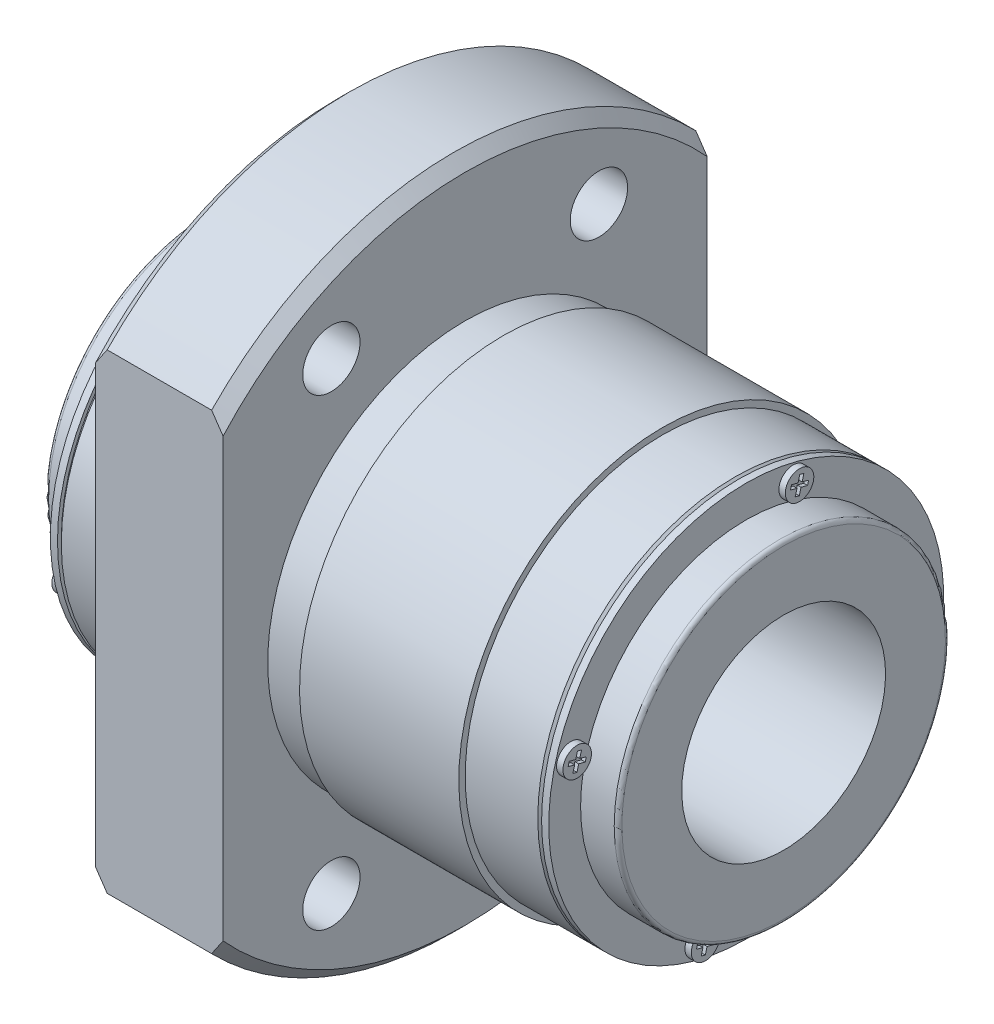
from build123d import *

# Parameters (mm, degrees)
SKETCH2_OUTSIDE_W          = 72.484
SKETCH2_OUTSIDE_H          = 72.484
SKETCH2_OUTSIDE_W_2        = 38
SKETCH2_OUTSIDE_H_2        = 53
CUT_EXTRUDE1_DEPTH         = 52.278650528
F_4_5_4_5_DIAMETER_HOLE1_D = 4.5
SKETCH6_R                  = 1.12
BOSS_EXTRUDE1_DEPTH        = 0.5
CUT_EXTRUDE2_DEPTH         = 0.3
CIRPATTERN1_COUNT          = 4
SKETCH8_R                  = 1.12
BOSS_EXTRUDE2_DEPTH        = 0.5
CUT_EXTRUDE3_DEPTH         = 0.3
CIRPATTERN2_COUNT          = 4
M6_TAPPED_HOLE1_D          = 5
M6_TAPPED_HOLE1_DEPTH      = 11
M6_TAPPED_HOLE1_TIP        = 1.502151548
CHAMFER1_SIZE              = 0.9
FILLET1_R                  = 0.3


with BuildPart() as part:
    # Sketch1 → Revolve1 (revolve)
    with BuildSketch(Plane.XY):
        Polygon((35, 8), (-10, 8), (-10, 13), (-7.06, 13), (-7.06, 15.5), (-0.65, 15.5), (-0.65, 16), (0, 16), (0, 26.5), (10, 26.5), (10, 15.5), (13, 15.5), (13, 16), (25.5, 16), (25.5, 15.5), (32.06, 15.5), (32.06, 13), (35, 13), align=None)
    revolve(axis=Axis((35, 0, 0), (-1, 0, 0)))

    # Sketch2 outside → Cut-Extrude1 (cut, through all)
    with BuildSketch(Plane(origin=(0, 0, 0), x_dir=(0, 0, -1), z_dir=(1, 0, 0))):
        Rectangle(SKETCH2_OUTSIDE_W, SKETCH2_OUTSIDE_H)
        Rectangle(SKETCH2_OUTSIDE_W_2, SKETCH2_OUTSIDE_H_2, mode=Mode.SUBTRACT)
    extrude(amount=CUT_EXTRUDE1_DEPTH, mode=Mode.SUBTRACT)

    # Ø4.5 (4.5) Diameter Hole1 (through all)
    with Locations(Plane(origin=(10, 0, 0), x_dir=(0, 0, -1), z_dir=(1, 0, 0))):
        with Locations((-10.5, 18.186533479), (-10.5, -18.186533479), (10.5, 18.186533479), (10.5, -18.186533479)):
            Hole(F_4_5_4_5_DIAMETER_HOLE1_D / 2)

    # Sketch6 → Boss-Extrude1 (add)
    with BuildSketch(Plane(origin=(32.06, 0, 0), x_dir=(0, 0, -1), z_dir=(1, 0, 0))):
        with Locations(Location((3.688171393, 13.764443025, 0), (0, 0, 90))):
            Circle(SKETCH6_R)
        with Locations(Location((-13.764443025, 3.688171393, 0), (0, 0, 90))):
            Circle(SKETCH6_R)
        with Locations(Location((-3.688171393, -13.764443025, 0), (0, 0, 90))):
            Circle(SKETCH6_R)
        with Locations(Location((13.764443025, -3.688171393, 0), (0, 0, 90))):
            Circle(SKETCH6_R)
    extrude(amount=BOSS_EXTRUDE1_DEPTH)

    # Sketch7 → Cut-Extrude2 (cut)
    with BuildSketch(Plane(origin=(32.56, 0, 0), x_dir=(0, 0, -1), z_dir=(1, 0, 0))):
        Polygon((4.02742839, 14.393056331), (3.708672868, 14.478466616), (3.571498774, 13.966525928), (3.059558086, 14.103700022), (2.974147801, 13.7849445), (3.486088489, 13.647770406), (3.348914395, 13.135829718), (3.667669918, 13.050419433), (3.804844012, 13.562360121), (4.3167847, 13.425186027), (4.402194984, 13.74394155), (3.890254296, 13.881115644), align=None)
    cut_extrude2 = extrude(amount=-CUT_EXTRUDE2_DEPTH, mode=Mode.SUBTRACT)

    # CirPattern1: Cut-Extrude2 ×4 about axis
    cirpattern1_axis = Axis((0, 0, 0), (1, 0, 0))
    for i in range(1, CIRPATTERN1_COUNT):
        add(cut_extrude2.rotate(cirpattern1_axis, i * 360 / CIRPATTERN1_COUNT), mode=Mode.SUBTRACT)

    # Sketch8 → Boss-Extrude2 (add)
    with BuildSketch(Plane.ZY.offset(7.06)):
        with Locations(Location((3.688171393, 13.764443025, 0), (0, 0, 270))):
            Circle(SKETCH8_R)
        with Locations(Location((-13.764443025, 3.688171393, 0), (0, 0, 270))):
            Circle(SKETCH8_R)
        with Locations(Location((-3.688171393, -13.764443025, 0), (0, 0, 270))):
            Circle(SKETCH8_R)
        with Locations(Location((13.764443025, -3.688171393, 0), (0, 0, 270))):
            Circle(SKETCH8_R)
    extrude(amount=BOSS_EXTRUDE2_DEPTH)

    # Sketch9 → Cut-Extrude3 (cut)
    with BuildSketch(Plane.ZY.offset(7.56)):
        Polygon((3.571498774, 13.966525928), (3.708672868, 14.478466616), (4.02742839, 14.393056331), (3.890254296, 13.881115644), (4.402194984, 13.74394155), (4.3167847, 13.425186027), (3.804844012, 13.562360121), (3.667669918, 13.050419433), (3.348914395, 13.135829718), (3.486088489, 13.647770406), (2.974147801, 13.7849445), (3.059558086, 14.103700022), align=None)
    cut_extrude3 = extrude(amount=-CUT_EXTRUDE3_DEPTH, mode=Mode.SUBTRACT)

    # CirPattern2: Cut-Extrude3 ×4 about axis
    cirpattern2_axis = Axis((0, 0, 0), (1, 0, 0))
    for i in range(1, CIRPATTERN2_COUNT):
        add(cut_extrude3.rotate(cirpattern2_axis, i * 360 / CIRPATTERN2_COUNT), mode=Mode.SUBTRACT)

    # M6 Tapped Hole1
    with Locations(Plane.XZ.offset(26.5)):
        with Locations((5, 0)):
            Hole(M6_TAPPED_HOLE1_D / 2, depth=M6_TAPPED_HOLE1_DEPTH)
            with Locations((0, 0, -(M6_TAPPED_HOLE1_DEPTH + M6_TAPPED_HOLE1_TIP / 2))):  # 118° drill point
                Cone(0, M6_TAPPED_HOLE1_D / 2, M6_TAPPED_HOLE1_TIP, mode=Mode.SUBTRACT)

    # Sketch12 → Cut-Revolve1 (revolve, cut)
    with BuildSketch(Plane(origin=(0, 0, 0), x_dir=(1, 0, 0), z_dir=(0, 1, 0)), mode=Mode.PRIVATE) as cut_revolve1_sk:
        Polygon((31.2, -15.5), (31.5, -15.2), (31.5, -15.5), align=None)
        Polygon((-6.5, -15.5), (-6.5, -15.2), (-6.2, -15.5), align=None)
    revolve(cut_revolve1_sk.sketch.rotate(Axis((-12.404699919, 0, 0), (1, 0, 0)), 270), axis=Axis((-12.404699919, 0, 0), (1, 0, 0)), mode=Mode.SUBTRACT)

    # Chamfer1
    chamfer1_edges = [part.edges().sort_by_distance(p)[0] for p in [
        (10, 26.5, 0),
        (0, 26.5, 0),
        (10, -26.5, 0),
        (0, -26.5, 0),
    ]]
    chamfer(chamfer1_edges, length=CHAMFER1_SIZE)

    # Fillet1
    fillet1_edges = [part.edges().sort_by_distance(p)[0] for p in [
        (35, -13, 0),
        (-10, -13, 0),
    ]]
    fillet(fillet1_edges, radius=FILLET1_R)


solid = part.part
